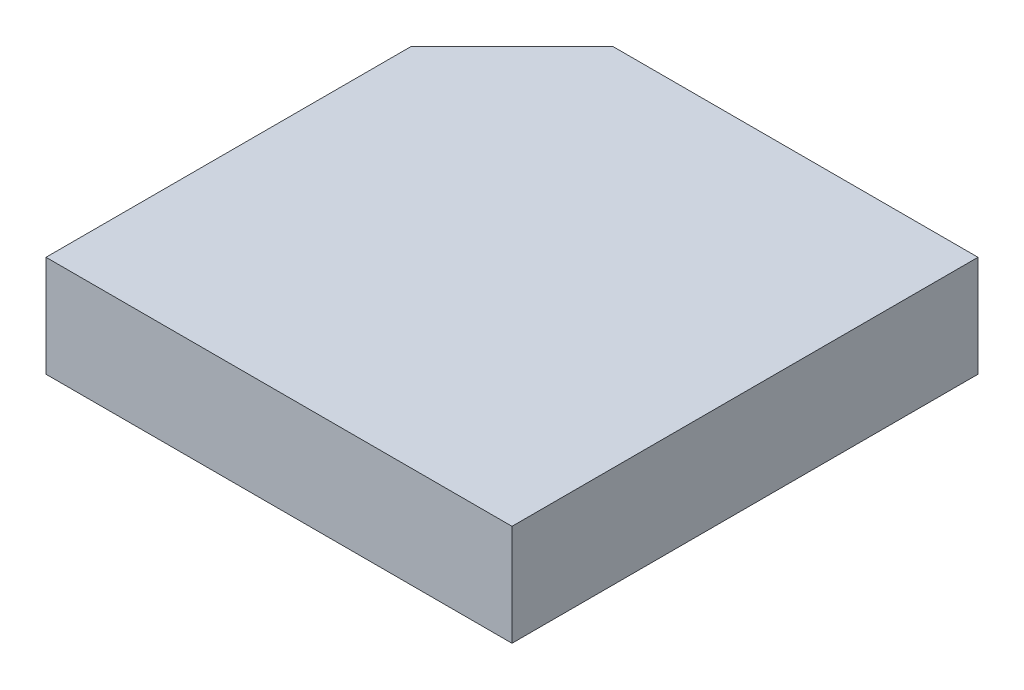
SolidWorks part; units mm, degrees
ref_plane "前视基准面" through (0, 0, 0) normal (0, 0, 1) x (1, 0, 0)
ref_plane "上视基准面" through (0, 0, 0) normal (0, 1, 0) x (1, 0, 0)
ref_plane "右视基准面" through (0, 0, 0) normal (1, 0, 0) x (0, 0, -1)
sketch "草图1" plane through (0, 0, 0) normal (0, 1, 0) x (1, 0, 0)
  line L0 (-115, 90) -> (-90, 115)
  line L1 (0, 0) -> (-115, 0)
  line L2 (0, 0) -> (0, 115)
  line L3 (0, 115) -> (-90, 115)
  line L4 (-115, 0) -> (-115, 90)
  dimension "D1" = 115
  dimension "D2" = 90
  dimension "D3" = 115
  dimension "D4" = 90
extrude "凸台-拉伸1" add sketch "草图1" along normal blind 25
